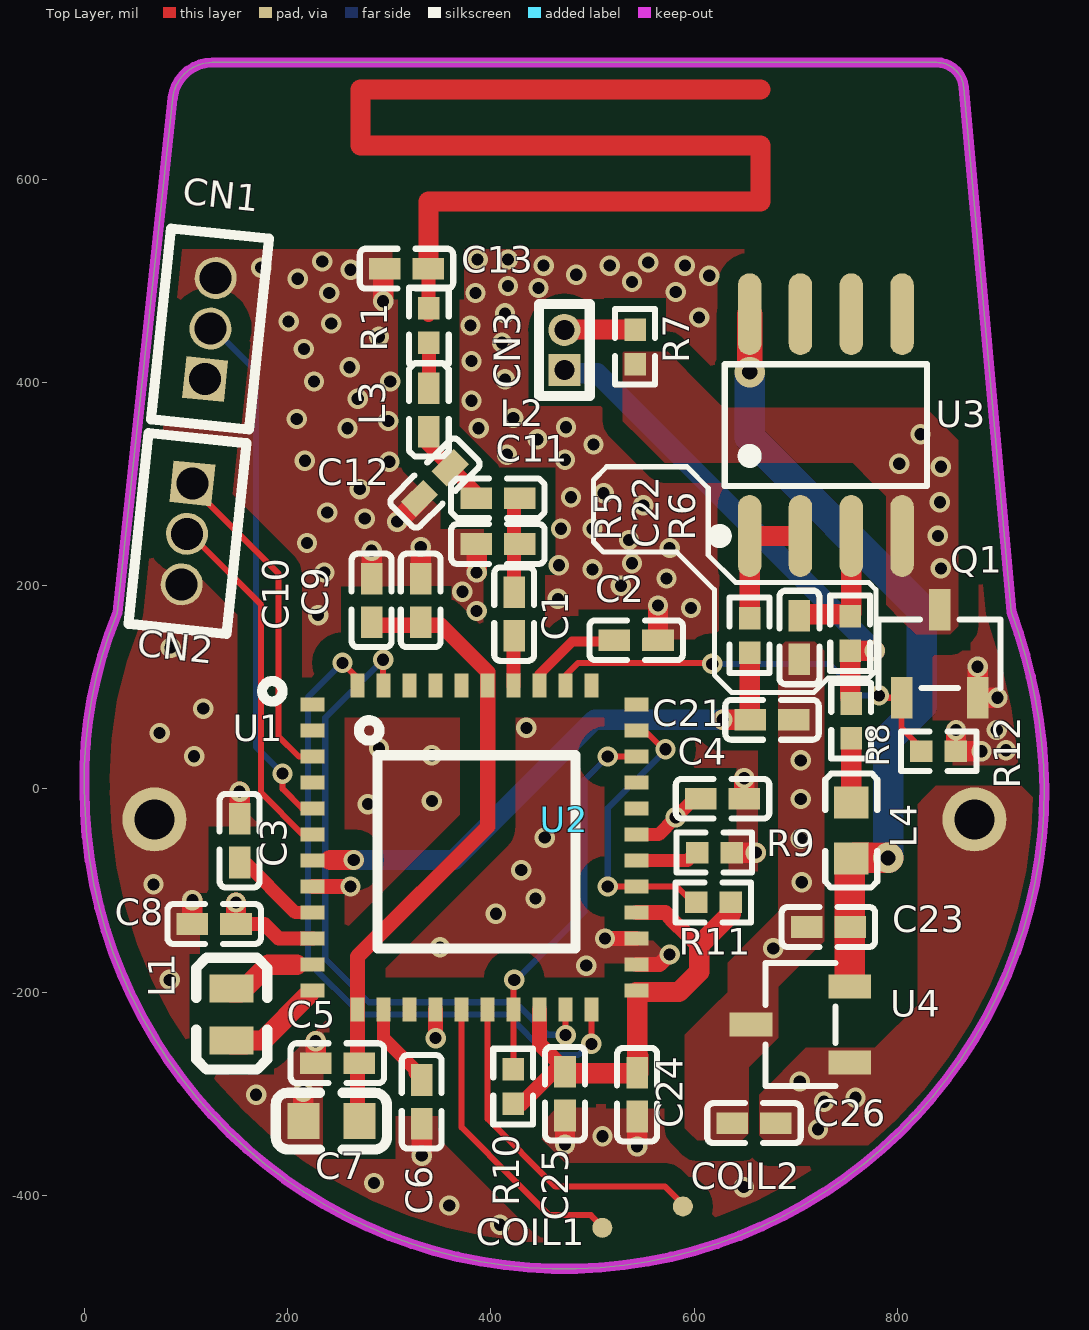
[diagram p0: Top Layer view]
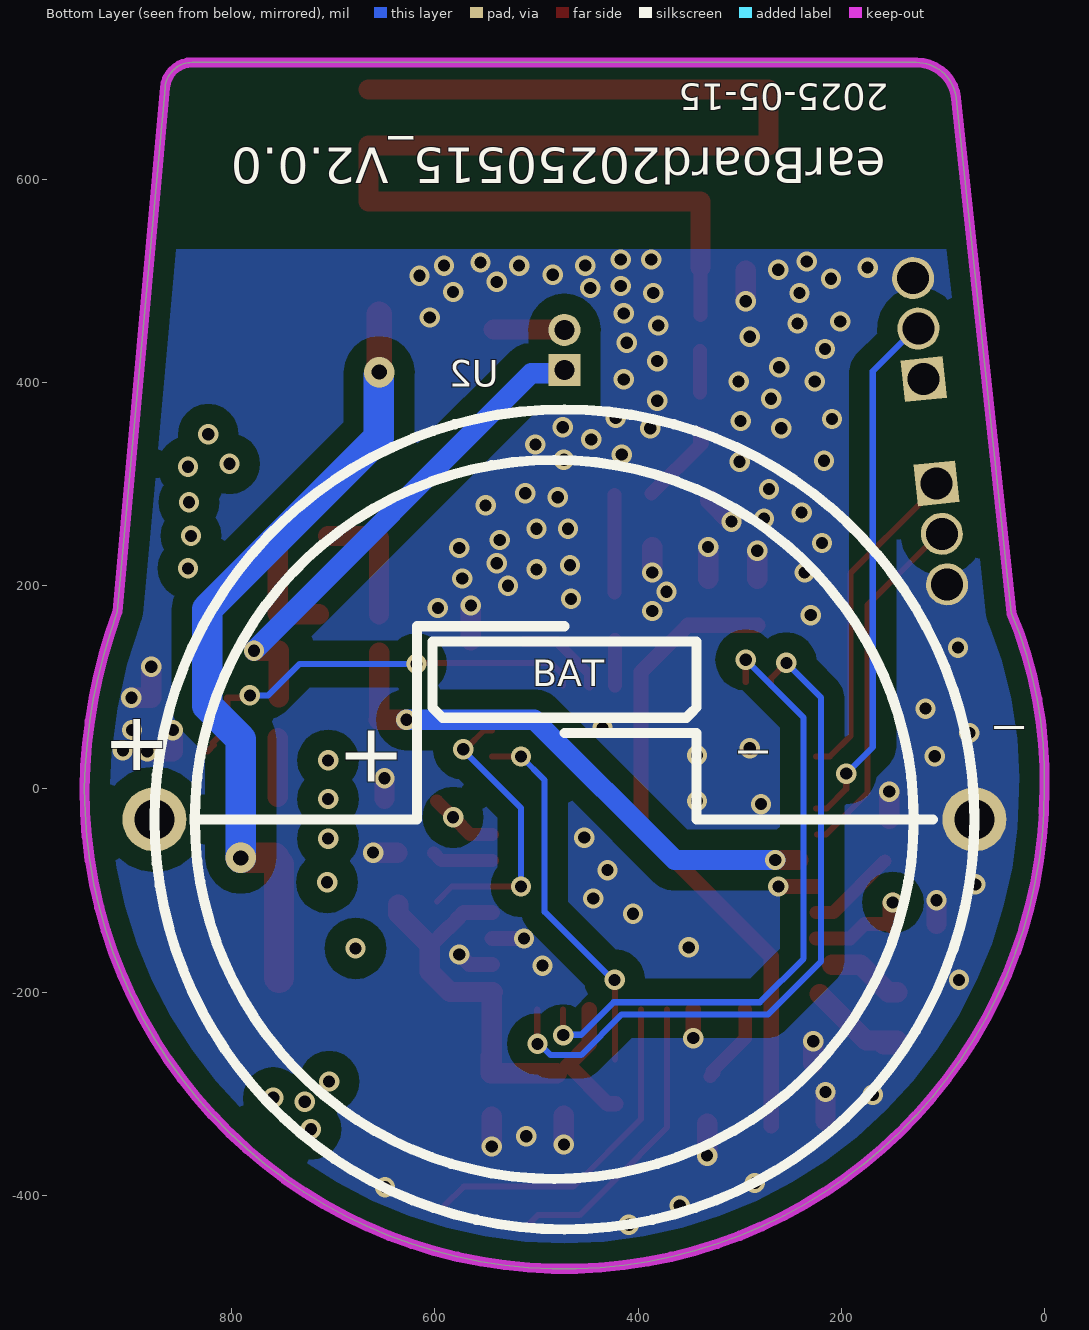
[diagram p1: Bottom Layer view, seen from below]
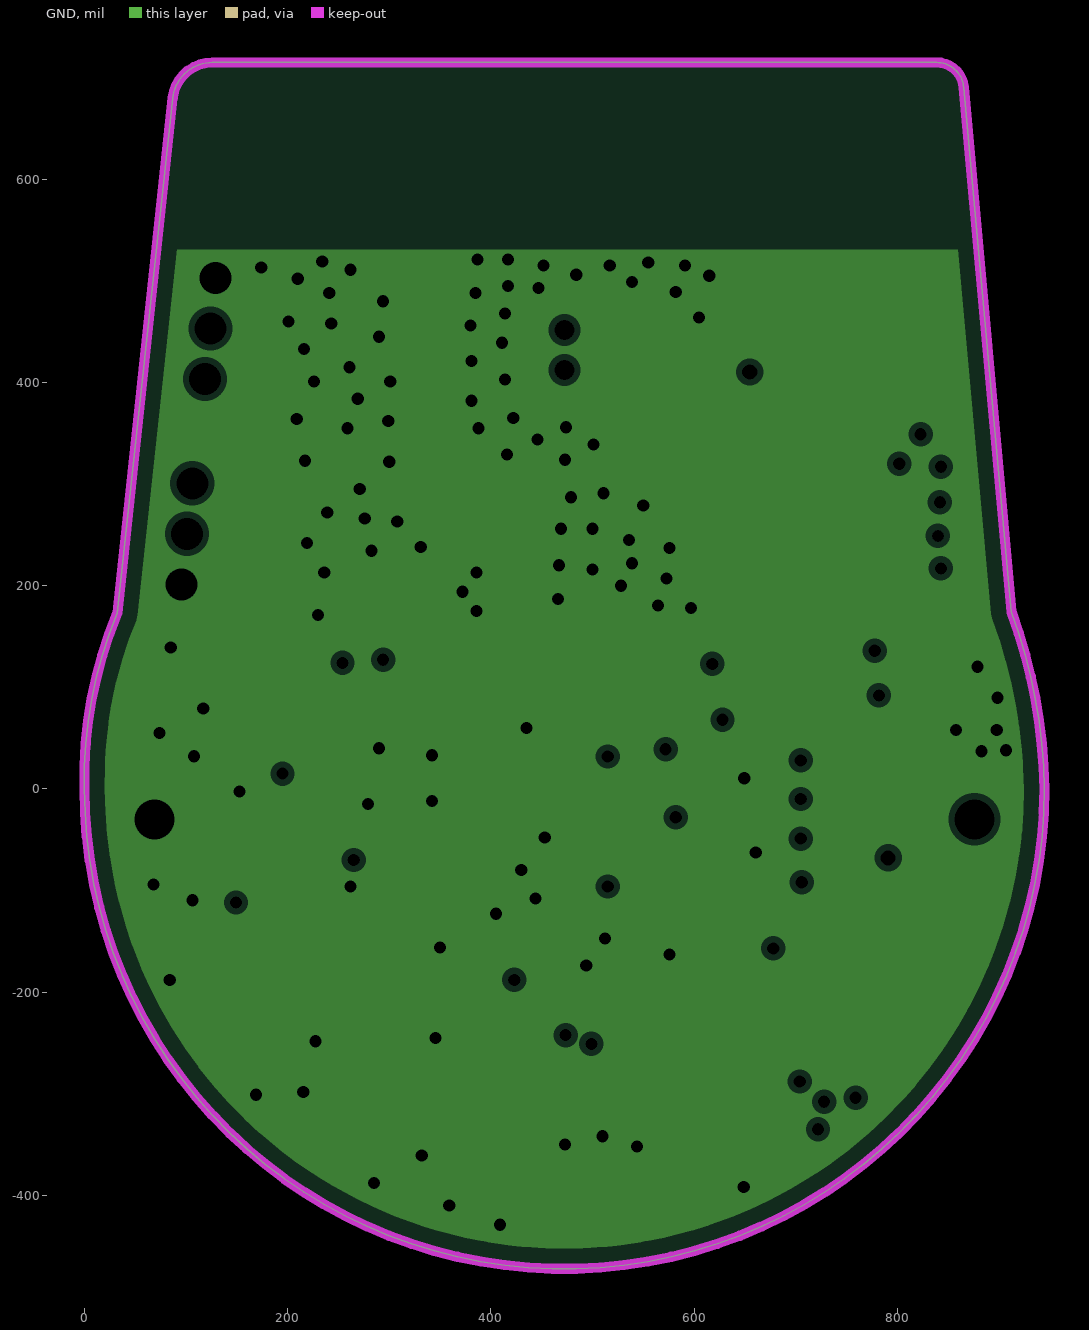
[diagram p2: GND, clearances drawn from the general rule]
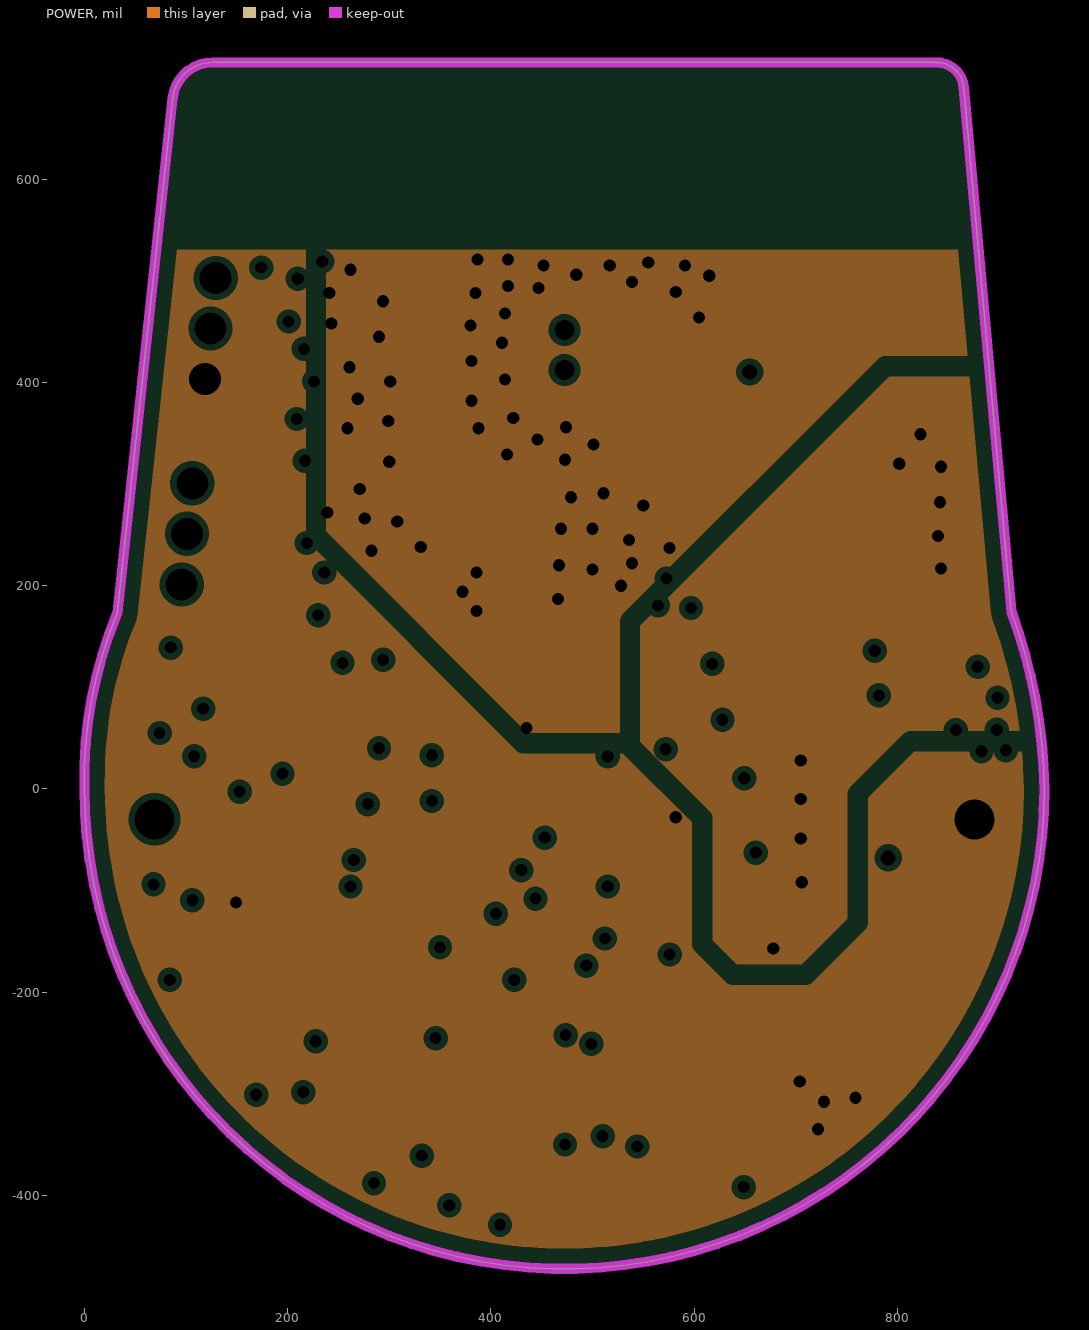
[diagram p3: POWER, clearances drawn from the general rule]
# Altium PCB MISC82703.PcbDoc
Units mil, origin at the board's own origin, x right, y up, seen from the top; angles counter-clockwise.
Board outline 944.88 x 1187.29 mil, 4 copper layers (Top Layer, GND, POWER, Bottom Layer); 42 components, 33 nets, 134 pads, 148 vias.

## Layer stack, top to bottom (the 12.6 mil dielectric is the usual default, probably not edited)
Top Layer: signal copper 1.4
Dielectric: core 12.6, FR-4, Dk 4.8
GND: plane copper 1.4, net GND
Dielectric: prepreg 12.6, FR-4, Dk 4.8
POWER: plane copper 1.4, net TL_VDD3
Dielectric: core 12.6, FR-4, Dk 4.8
Bottom Layer: signal copper 1.4

## Board outline
0,0 cw(c423.07,10.33) 32.44,173.13 86.87,679.84 cw(c126.01,675.63) 126.01,715 838.85,715 cw(c838.85,688.3) 865.48,690.34 912.44,174.28 912.44,174.29 cw(c411.43,-9.13) 944.88,0 cw(c472.44,0)

## Design rules (kind name [scope] priority, off if disabled: settings)
Clearance Clearance_1 [inpolygon] p1: gap=6
Clearance [All] p2: gap=6
DiffPairsRouting [All] p1: maxlimit=6 minlimit=6 mostfreqgap=6 maxuncoupledlength=500
HoleSize [All] p1: absolutevalues=TRUE maxlimit=500 minlimit=1 maxpercent=80.000 minpercent=20.000
HoleToHoleClearance [All] p1: gap=0 allowstackedmicrovias=TRUE
MinimumSolderMaskSliver [All] p1: minsoldermaskwidth=0
PlaneClearance [All] p1: clearance=6
PlaneConnect [All] p1: planeconnectstyle=Direct reliefexpansion=20 reliefentries=4 reliefconductorwidth=10 reliefairgap=10
PolygonConnect [All] p1: connectstyle=Direct reliefconductorwidth=10 reliefentries=4 polygonreliefangle="90 Angle"
RoutingVias [All] p1: holewidth=12 width=20 viastyle="Through Hole" minholewidth=12 minwidth=20 maxholewidth=12 maxwidth=20
SilkToSilkClearance [All] p1: silktosilkclearance=0
SilkscreenOverComponentPads [All] p1: minsilkscreentomaskgap=0
SolderMaskExpansion [All] p1: expansion=4
Width [All] p1: maxlimit=40 minlimit=6 preferedwidth=10
20 further rules are at their usual default settings.

## Classes and differential pairs
component class 1_Power电源管理+天线+加速度: C1 C2 C3 C4 C5 C6 C7 C8 C9 C10 C11 C12 C13 C24 C25 CN1 CN2 COIL1 COIL2 L1 L2 L3 R1 R9 R10 R11 U1 U2
component class 2_温度采集: C21 C22 C23 C26 CN3 L4 Q1 R5 R6 R7 R8 R12 U3 U4

## Components (designator, comment, footprint, x,y, rotation, side; value= is the part's Value field where it differs from the comment)
C1 "220pF" C0402 423,172 r90 top
C2 "1uF" C0402 543.07,146.26 r180 top
C3 "1uF" C0402 152.74,-50.99 r270 top
C4 "1uF" C0402 628.07,-9.74 r180 top
C5 "1uF" C0402 249,-270 r0 top
C6 "1uF" C0402 332,-308 r90 top
C7 "0.1uF" C0603 243,-327 r0 top
C8 "1uF" C0402 127.74,-132.99 r180 top
C9 "2.2uF" C0402 331,185.46 r270 top
C10 "0.1uF" C0402 282.7,185.45 r270 top
C11 "2pF" C0402 407,241 r0 top
C12 "2pF" C0402 345,301 r45 top
C13 "2pF" C0402 317,512 r0 top
C21 "10pF" C0402 676.74,68.01 r180 top
C22 "100nF" C0402 703.74,149.01 r90 top
C23 "100nF" C0402 732.25,-135.92 r180 top
C24 "0.1uF-c0402" C0402 544,-301 r270 top
C25 "0.1uF-c0402" C0402 473,-300 r270 top
C26 "470nF" C0402 659,-329 r0 top
CN1 "" HDR-TH_3P-P1.27-V-M-A 124,453 r84 top
CN2 "" HDR-TH_3P-P1.27-V-M-A 101,251 r264 top
CN3 "HX PZ1.0-1x2P ZZ" HDR-TH_2P-P1.00-V-M 472.44,432.01 r90 top
COIL1 "" Test-Point-0.5mm 509.74,-431.99 r0 top
COIL2 "" Test-Point-0.5mm 589,-411 r0 top
L1 "4.7uH" IND-SMD_L1.8-W1.2 145,-222 r90 top
L2 "2.4nH" L0402 407,286 r180 top
L3 "2.4nH" L0402 339,373 r90 top
L4 "MPZ1608S101ATAH0" L0603 754.74,-40.99 r270 top
Q1 "BSS138" SOT-23-3_L3.0-W1.7-P0.95-LS2.9-BR 841.74,133.01 r270 bottom
R1 "" R0402 339,456 r90 top
R5 "" R0402 654.74,151.01 r90 top
R6 "" R0402 753.74,153.01 r90 top
R7 "" R0402 542,435 r90 top
R8 "" R0402 754.74,67.01 r270 top
R9 "" R0402 620.07,-62.74 r180 top
R10 "" R0402 422,-293 r270 top
R11 "" R0402 619.07,-111.74 r0 top
R12 "" R0402 840.74,37.01 r180 top
U1 "" KTYATR0101 384.07,-57.74 r0 top
U2 "Q&J CR2032 20-6*9" BAT-TH_CR2032 472.44,-30 r180 top locked
U3 "MCP6022-I/SN" SOIC-8_L4.9-W3.9-P1.27-LS6.0-BL 729.74,358.01 r0 top
U4 "REF3025AIDBZR" SOT-23-3_L2.9-W1.6-P1.90-LS2.8-BR 704.74,-231.99 r0 bottom

## Footprints (in the part's own frame and the unit in brackets; to place one, negate y for a bottom-side part, rotate by r counter-clockwise, add the part's x,y. Pads: shape width x height; smd on the part's side, far side on the other; paste and mask are expansions set on the pad)
BAT-TH_CR2032 [mm]
  round 1.6 hole 1: 1(-10.25,0) 2(10.25,0)
C0402 [mm]
  rect 0.79x0.54 smd paste-100 mask+0.051: 1(-0.545,0) 2(0.545,0)
  silkscreen extent -1.17,-0.5 1.17,0.5
C0603 [mm]
  rect 0.8x0.9 smd: 1(-0.7,0) 2(0.7,0)
  silkscreen extent -1.39,-0.71 1.39,0.71
HDR-TH_2P-P1.00-V-M [mm]
  rect 0.8x0.8 hole 0.5 paste+0 mask+0.05: 1(-0.5,0)
  round 0.8 hole 0.5 paste+0 mask+0.05: 2(0.5,0)
  silkscreen extent -1.15,-0.64 1.15,0.64
HDR-TH_3P-P1.27-V-M-A [mm]
  rect 1.05x1.05 hole 0.8: 1(-1.27,0)
  round 1.05 hole 0.8: 2(0,0) 3(1.27,0)
  silkscreen extent -2.41,-1.22 2.39,1.24
IND-SMD_L1.8-W1.2 [mm]
  rect 0.7x1.1 smd: 1(-0.653,0) 2(0.653,0)
  silkscreen extent -1.38,-0.89 1.41,0.89
KTYATR0101 [mm]
  rect 0.6x0.35 smd: 1(-4.05,3.575) 2(-4.05,2.925) 3(-4.05,2.275) 4(-4.05,1.625) 5(-4.05,0.975) 6(-4.05,0.325) 7(-4.05,-0.325) 8(-4.05,-0.975) 9(-4.05,-1.625) 10(-4.05,-2.275) 11(-4.05,-2.925) 12(-4.05,-3.575) 23(4.05,-3.575) 24(4.05,-2.925) 25(4.05,-2.275) 26(4.05,-1.625) 27(4.05,-0.975) 28(4.05,-0.325) 29(4.05,0.325) 30(4.05,0.975) 31(4.05,1.625) 32(4.05,2.275) 33(4.05,2.925) 34(4.05,3.575)
  rect 0.35x0.6 smd: 13(-2.925,-4.05) 14(-2.275,-4.05) 15(-1.625,-4.05) 16(-0.975,-4.05) 17(-0.325,-4.05) 18(0.325,-4.05) 19(0.975,-4.05) 20(1.625,-4.05) 21(2.275,-4.05) 22(2.925,-4.05) 35(2.925,4.05) 36(2.275,4.05) 37(1.625,4.05) 38(0.975,4.05) 39(0.325,4.05) 40(-0.325,4.05) 41(-0.975,4.05) 42(-1.625,4.05) 43(-2.275,4.05) 44(-2.925,4.05)
  silkscreen extent -5.31,-2.52 2.53,4.16
L0402 [mm]
  rect 0.79x0.54 smd paste-100 mask+0.051: 1(-0.545,0) 2(0.545,0)
  silkscreen extent -1.17,-0.5 1.17,0.5
L0603 [mm]
  rect 0.8x0.864 smd paste-100 mask+0.051: 1(-0.7,0) 2(0.7,0)
  silkscreen extent -1.42,-0.65 1.42,0.65
R0402 [mm]
  rect 0.566x0.54 smd paste-100 mask+0.051: 1(-0.433,0) 2(0.433,0)
  silkscreen extent -0.94,-0.5 0.94,0.5
SOIC-8_L4.9-W3.9-P1.27-LS6.0-BL [mm]
  oval 0.588x2.045 smd: 1(-1.905,-2.772) 2(-0.635,-2.772) 3(0.635,-2.772) 4(1.905,-2.772) 5(1.905,2.772) 6(0.635,2.772) 7(-0.635,2.772) 8(-1.905,2.772)
  silkscreen extent -2.8,-2.92 2.53,1.52
SOT-23-3_L2.9-W1.6-P1.90-LS2.8-BR [mm]
  rect 1.07x0.6 smd far side: 1(1.235,0.95) 2(1.235,-0.95) 3(-1.235,0)
SOT-23-3_L3.0-W1.7-P0.95-LS2.9-BR [mil]
  rect 40.85x20.95 smd far side: 1(43.36,37.4) 2(43.36,-37.4) 3(-43.36,0)
Test-Point-0.5mm [mm]
  round 0.5 smd: 1(0,0)

## Part data
C1: library part CC0402KRX7R9BB221
C2 C3 C4 C5 C6 C8 C9 C10: library part CL05A105KA5NQNC
C7: library part CAP_0603
C11 C12 C13: library part CC0402CRNPO9BN2R0
C21: library part CC0402JRNPO9BN100
C22 C23: library part GRM155R71H104KE14D
C26: library part CGA0402X7R474K100GT
CN1 CN2: library part 3Pin_1.27___
COIL1 COIL2: library part Test-Point
L1: library part SLC1608F4R7KTT
L2 L3: library part LQG15HH2N4S02D
R1: library part SCR0402J0R
R5: library part RC0402FR-0733RL
R6 R7: library part RT0402BRD0710KL
R8: library part RT0402BRD07100KL
R9 R10 R11: library part 0402WGF4701TCE
R12: library part 0402WGF1002TCE
U1: library part KTYATR0101

## Via types
v1: diameter 20, hole 12, Top Layer to Bottom Layer, tented bottom, 105 vias
v2: diameter 20, hole 12, Top Layer to Bottom Layer, 41 vias
v3: diameter 30, hole 15, Top Layer to Bottom Layer, tented bottom, 2 vias

## Nets (pads, with @x,y where several pads share a name; then routed paths per layer and width w, separated by ;. In a path a pad name is that pad's centre, name@x,y a point inside that pad or via, vN(x,y) a via of type N, cw(c..) or ccw(c..) an arc to the next point about the centre after c; other vN are vias at no path point)
ANT: C1.1 U1.38 | length 44.8
  Top Layer w13.75: U1.38 C1.1@422.45,146.55
ANTENNA: C13.2 R1.2 | length 1334.8
  Top Layer w13.75: R1.2@338.46,466.54 C13.2
  Top Layer w19.68: C13.2@338.51,513.26 338.51,578.22 665.29,578.22 665.29,633.34 271.59,633.34 271.59,688.46 665.29,688.46
GND: C2.1 C3.1 C4.1 C5.1 C6.1 C7.1 C8.2 C9.1 C10.1 C11.1 C12.1 C13.1 C24.2 C25.2 CN1.3 CN2.3 Q1.2 R9.1 R12.1 U1.8 U1.16 U1.24 U1.25 U2.2 | length 640.2
  Top Layer w15: U1.8 v1(261.88,-96.12) ; v1(345.68,-245.32) U1.16 ; v1(512.3,-147.3) U1.25 ; U1.24 566.1,-172.9 v1(576,-163)
  Top Layer w20: C8.2 v1(106.28,-109.72) ; C3.1 v1(152.74,-2.74) ; C7.1 v1(215.44,-298.44) ; C5.1 v1(227.54,-248.46) ; C10.1 v1(282.7,234.3) ; v1(294,480) C13.1@294,510 ; v1(308,263) C12.1@329,284 ; C9.1 v1(331,238) ; v1(332,-361) C6.1 ; v1(386,213) C11.1@386,238 ; v1(473,-350) C25.2 ; v1(544,-352) C24.2 ; C2.1 v1(564.53,180.47) ; R9.1 v1(660.74,-62.74) ; C4.1 v1(649.53,10.53) ; v1(857.78,57.78) R12.1 v1(882.99,37.01) ; v1(879.14,120.14) Q1.2 v1(898.65,89.65)
  other v1: 409,-429 359,-410 649,-392 285,-388 510,-342 169,-301 84,-188 494,-174 350,-156 405,-123 444,-108 68,-94 430,-80 453,-48 279,-15 342,-12 108,32 342,33 907,38 290,40 74,55 898,58 435,60 117,79 85,139 230,171 386,175 597,178 466,187 372,194 528,200 236,213 576,237 536,245 469,256 239,272 550,279 511,291 300,322 217,323 259,355 299,362 226,401 301,401 243,458 201,460 605,464 210,502 452,515 517,515 591,515
  other v2: 573,207 500,216 467,220 539,222 219,242 500,256 276,266 479,287 271,295 473,324 416,329 501,339 446,344 388,355 474,356 209,364 422,365 381,382 269,384 414,403 261,415 381,421 216,433 411,439 290,445 380,456 414,468 241,488 385,488 582,489 447,493 417,495 539,499 615,505 484,506 262,511 174,513 555,518 234,519 387,521 417,521
NetC1_2: C1.2 C11.2 L2.1 | length 95.5
  Top Layer w13.75: C1.2 L2.1@423,289
NetC3_2: C3.2 U1.9 | length 88.6
  Top Layer w13: C3.2@157,-71 207.71,-121.71 U1.9
NetC12_2: C12.2 L2.2 L3.1 | length 76.5
  Top Layer w13.75: L3.1@337,340 L2.2@386.5,290.5 ; L3.1@339,343 L3.1@339,349.54
NetC21_1: C21.1 C22.1 C23.2 C26.1 Q1.3 R7.1 U3.4 U4.3
  other v1: 678,-157 706,-92 705,-49 705,-10 705,28 843,217 840,249 842,282 843,317 802,320 823,349
NetC22_2: C22.2 R6.2 U3.3 | length 117.2
  Top Layer w20: C22.2@714,172 754,172 754.74,172.74 U3.3
NetC23_1: C23.1 L4.2 U3.8 U4.2 | length 766.2
  Top Layer w20: L4.2@753.37,-74.63 L4.2@753.37,-71.63
  Top Layer w25: v3(654.74,410.26) U3.8
  Top Layer w30: U4.2@753.37,-186 L4.2@753.37,-74.63 ; L4.2@758,-68 v3(791,-68)
  Bottom Layer w20: v3@654.74,407 v3(654.74,410.26)
  Bottom Layer w30: v3@655,407 655,346 824,177 824,82 791,49 v3(791,-68)
NetCN3_1: CN3.1 R6.1 R8.1 | length 482
  Top Layer w20: R8.1@753.74,90.26 R6.1 v1(777.97,135.97)
  Bottom Layer w20: CN3.1@479,409 504.94,409 v1(777.97,135.97)
NetCN3_2: CN3.2 R7.2 | length 68
  Top Layer w20: CN3.2@474.04,452.04 R7.2
NetCOIL1_1: COIL1.1 U1.17 | length 296.7
  Top Layer w6: U1.17 371.27,-333.27 425,-387 457.5,-419.5 498.5,-419.5 COIL1.1@511,-432
NetCOIL2_1: COIL2.1 U1.18 | length 336.1
  Top Layer w6: U1.18 396.86,-324.86 463.5,-391.5 571.5,-391.5 COIL2.1@590,-410
NetL1_1: L1.1 U1.12 | length 108.2
  Top Layer w20: L1.1@145,-251.69 L1.1@158.31,-251.69 ; L1.1 175.31,-247.69 U1.12@221,-202
NetL1_2: L1.2 U1.11 | length 75.3
  Top Layer w20: L1.2@145,-200.31 153.69,-200.31 181,-173 209,-173
NetL3_2: L3.2 R1.1 | length 41
  Top Layer w13.75: L3.2@339,390 R1.1@339,430.96
NetL4_1: L4.1 R8.2 | length 57.7
  Top Layer w20: L4.1@754.74,-7.74 R8.2
NetR5_2: R5.2 U3.1 U3.2 | length 125.3
  Top Layer w20: R5.2@655,172 655,246.72 657.14,248.86 U3.2
NetR9_2: R9.2 U1.28 | length 60.6
  Top Layer w13: U1.28 593.47,-70.53 R9.2@601,-63
PD3: U1.21 U1.43 | length 632.6
  Top Layer w6: U1.43@294,105 v1(294,127) ; v1(473.64,-242.36) U1.21
  Bottom Layer w6: v1(294,127) 237,70 237,-167 280,-210 424,-210 456,-242 v1@473,-242 ; v1@473.14,-241.86 v1(473.64,-242.36)
PD4: U1.22 U1.44 | length 688.6
  Top Layer w6: v1(254,124) 268.91,109.09 U1.44 ; v1@499.21,-251 U1.22
  Bottom Layer w6: v1(254,124) 220,90 220,-170 272,-222 416,-222 456,-262 486,-262 v1@496,-252
  other v1: 499,-251
PGS: Q1.1 R12.2 U1.36 | length 420.6
  Top Layer w6: U1.36 473.64,111.64 486,124 v1@617,124 ; v1@780.35,89.65 Q1.1 804.34,59.66 R12.2@819,45 ; v1@780.35,92 v1(782,92) ; R12.2@817.36,43.36 R12.2
  Bottom Layer w6: v1(618,123) 733,123 764,92 v1(782,92)
RX: CN2.2 U1.6 | length 338.2
  Top Layer w6: CN2.2@113,242 174,181 174,-4 215,-45 U1.6@224,-45
SCL_ACC: R11.1 U1.27 U1.33 | length 285
  Top Layer w6: v1(515.12,-96.12) U1.27 583.12,-96.12 R11.1@598,-111 ; U1.33 551.58,57.42 568,41 v1@574,41
  Bottom Layer w6: v1(515.12,-96.12) 515.12,-18.88 572,38 v1(572,39)
SDA_ACC: R10.1 U1.19 U1.32 | length 359.9
  Top Layer w6: R10.1@422.45,-266.45 U1.19 v1@422.45,-193.55 ; v1(515.17,31.83) U1.32
  Bottom Layer w6: v1(423,-188) v1@426,-185 ; v1@427,-186 492,-121 492,8.66 v1(515.17,31.83)
TEMPA: C21.2 R5.1 U1.7 | length 530.7
  Top Layer w20: 242,-70 v1(265,-70) ; v1(628.01,68.01) C21.2 ; C21.2@654.74,73.74 R5.1
  Bottom Layer w20: v1(265,-70) 364,-70 502.01,68.01 v1(628.01,68.01)
TL_1V4: C5.2 C7.2 C9.2 C10.2 U1.13 U1.39 | length 634
  Top Layer w15: C7.2@268.91,-331.91 U1.13 268.91,-165.09 397,-37 397,115 351,161 C10.2@282,161
TL_RST: C2.2 U1.37 | length 88.5
  Top Layer w10: U1.37 448.05,113.05 480,145 C2.2@512,145
TL_SWS_A7: CN1.2 U1.5 | length 612.1
  Top Layer w6: v1(195,15) 195,0 214.35,-19.35 U1.5
  Bottom Layer w6: CN1.2@136,444 169,411 169,95 ; 169,201 169,95 ; v1(195,15) 169,41 169,95
TL_VDD3: C4.2 C8.1 C26.2 CN1.1 U1.10 U1.29 U2.1 U4.1 | length 166.3
  Top Layer w13: U1.29 565.06,-44.94 v1@581,-29 ; v1(582,-28) v1@581,-29 ; C4.2@598,-12 v1@581,-29
  Top Layer w14: C8.1@155,-133 177,-133 191.3,-147.3 U1.10
  Top Layer w20: C8.1 v1(149.2,-111.8)
  other v1: 722,-335 728,-308 759,-304 704,-288
TX: CN2.1 U1.3 | length 303.8
  Top Layer w6: CN2.1@119,284 191,212 191,52 211.17,31.83 U1.3
VDD_1V8: C6.2 U1.14 | length 79.4
  Top Layer w13: U1.14 294.5,-245.5 C6.2@327,-278 ; U1.14@295,-217.19 U1.14@295,-217 ; C6.2@325.5,-279.5 C6.2@329,-283
VDD_ACC: C24.1 C25.1 R10.2 R11.2 U1.20 U1.23 U1.26 | length 509.4
  Top Layer w15: R10.2 429.96,-310.04 467,-273 470,-273 448.05,-251.05 U1.20 ; U1.26 571.71,-121.71 577.39,-127.39 577.39,-127.96 585.3,-135.87 585.87,-135.87 605,-155
  Top Layer w20: C25.1@480,-280 543,-280 544,-279 U1.23@544,-204 ; U1.23@543,-200 585,-200 605,-180 605,-155 605,-154 636,-123 R11.2@636,-114 ; C24.1@545,-280 545,-263
pads on no net: U1.1 U1.2 U1.4 U1.15 U1.30 U1.31 U1.34 U1.35 U1.40 U1.41 U1.42 U3.5 U3.6 U3.7

## Polygon pours and split planes (outlines as drawn)
NetC21_1 on Top Layer "Bottom Layer-No Net" (solid, remove dead copper, pour order 1000): 591,-276 591,-334 596,-339 603,-346 615,-346 647,-346 652,-341 654,-339 654,-332 654,-274 679,-249 683,-245 683,-225 683,-195 723,-155 728,-150 728,-133 728,136 722,142 719,145 708,145 690,145 684,139 683,138 683,77 683,-121 654,-150 633,-171 633,-190 633,-200 618,-215 591,-242 591,-276
NetC21_1 on Top Layer "Bottom Layer-No Net" (solid, remove dead copper, pour order 1001): 530,416 530,362 548,344 571,321 653,321 756,321 777,300 789,288 789,265 789,181 805,165 818,152 839,152 852,152 858,158 860,160 860,166 860,343 827,376 826,375 695,375 629,375 611,393 574,430 551,430 531,430 530,429 530,416
TL_VDD3 on Top Layer "Bottom Layer-No Net" (solid, remove dead copper, pour order 1002): 664,-302 664,-341 670,-347 674,-351 697,-351 865,-351 903,-313 952,-264 952,-221 952,-27 923,2 922,3 903,3 838,3 827,-8 820,-15 820,-32 820,-213 781,-252 778,-255 747,-255 710,-255 664,-301
GND on Top Layer "Bottom Layer-No Net" (solid, remove dead copper, pour order 1003): -122.43,396.1 -116.43,390.1 -116.43,-499.9 967.57,-499.9 1060.57,-406.9 1131.57,-335.9 1131.57,-307.9 1131.57,757.1 1054.57,834.1 984.57,904.1 744.57,904.1 46.57,904.1 -58.43,799.1 -113.43,744.1 -113.43,415.1
GND on Bottom Layer "Bottom Layer-No Net" (solid, remove dead copper, pour order 1004): -171.87,446.8 -171.87,-330.2 -100.87,-401.2 8.13,-510.2 337.13,-510.2 883.13,-510.2 970.13,-423.2 1063.13,-330.2 1063.13,-324.2 1063.13,865.8 983.13,945.8 945.13,983.8 881.13,983.8 4.13,983.8 -132.87,846.8 -161.87,817.8 -161.87,436.8
GND on GND (split plane): 892.43,172.46 892.54,171.88 892.57,171.28 892.68,170.83 892.73,170.37 893,169.49 893.17,168.59 893.39,168.04 893.54,167.46 893.82,166.86 899.83,149.55 905.68,130.26 910.77,110.75 915.09,91.05 918.64,71.2 921.4,51.22 923.38,31.16 924.56,11.03 924.79,-0.34 924.82,-0.34 924.86,-0.78 924.49,-18.69 923.33,-37.36 921.4,-55.96 918.71,-74.47 915.25,-92.84 911.03,-111.06 906.07,-129.09 900.36,-146.9 893.93,-164.46 886.77,-181.74 878.91,-198.71 870.35,-215.33 861.11,-231.59 851.21,-247.46 840.66,-262.9 829.48,-277.89 817.69,-292.41 805.31,-306.43 792.36,-319.92 778.87,-332.87 764.85,-345.25 750.33,-357.03 735.34,-368.21 719.9,-378.76 704.04,-388.67 687.78,-397.9 671.15,-406.46 654.18,-414.33 636.91,-421.48 619.35,-427.92 601.54,-433.63 583.51,-438.59 565.29,-442.81 546.91,-446.26 528.4,-448.96 509.8,-450.89 491.14,-452.05 472.44,-452.43 453.74,-452.05 435.08,-450.89 416.48,-448.96 397.97,-446.26 379.59,-442.81 361.37,-438.59 343.34,-433.63 325.53,-427.92 307.98,-421.48 290.7,-414.33 273.73,-406.46 257.1,-397.9 240.84,-388.67 224.98,-378.76 209.54,-368.21 194.55,-357.03 180.03,-345.25 166.01,-332.87 152.52,-319.92 139.57,-306.43 127.19,-292.41 115.4,-277.89 104.23,-262.9 93.68,-247.46 83.77,-231.59 74.53,-215.33 65.97,-198.71 58.11,-181.74 50.95,-164.46 44.52,-146.9 38.81,-129.09 33.85,-111.06 29.63,-92.84 26.17,-74.47 23.48,-55.96 21.55,-37.36 20.39,-18.69 20.02,-0.78 20.1,0 20.05,0.49 20.09,0.49 19.88,10.33 20.26,27.92 21.41,45.47 23.33,62.96 26,80.35 29.44,97.6 33.62,114.69 38.54,131.57 44.19,148.23 50.49,164.43 50.84,165.04 50.96,165.42 50.99,165.4 51.01,165.44 51.27,166.3 51.62,167.13 51.79,167.97 52.06,168.78 52.09,169 52.15,169.21 52.24,170.11 52.42,170.99 91.09,531 859.8,531
TL_VDD3 on POWER (split plane): 217.91,249 218.26,246.39 219.26,243.96 220.87,241.87 424.87,37.87 426.96,36.26 429.39,35.26 432,34.91 529.83,34.91 529.87,34.87 597.91,-33.18 597.91,-153 598.26,-155.61 599.26,-158.04 600.87,-160.13 630.87,-190.13 632.96,-191.74 635.39,-192.74 638,-193.09 710,-193.09 712.61,-192.74 715.04,-191.74 717.13,-190.13 768.13,-139.13 769.73,-137.04 770.74,-134.61 771.09,-132 771.09,-9.18 817.18,36.91 922.81,36.91 923.38,31.16 924.56,11.03 924.79,-0.34 924.82,-0.34 924.86,-0.78 924.49,-18.69 923.33,-37.36 921.4,-55.96 918.71,-74.47 915.25,-92.84 911.03,-111.06 906.07,-129.09 900.36,-146.9 893.93,-164.46 886.77,-181.74 878.91,-198.71 870.35,-215.33 861.11,-231.59 851.21,-247.46 840.66,-262.9 829.48,-277.89 817.69,-292.41 805.31,-306.43 792.36,-319.92 778.87,-332.87 764.85,-345.25 750.33,-357.03 735.34,-368.21 719.9,-378.76 704.04,-388.67 687.78,-397.9 671.15,-406.46 654.18,-414.33 636.91,-421.48 619.35,-427.92 601.54,-433.63 583.51,-438.59 565.29,-442.81 546.91,-446.26 528.4,-448.96 509.8,-450.89 491.14,-452.05 472.44,-452.43 453.74,-452.05 435.08,-450.89 416.48,-448.96 397.97,-446.26 379.59,-442.81 361.37,-438.59 343.34,-433.63 325.53,-427.92 307.98,-421.48 290.7,-414.33 273.73,-406.46 257.1,-397.9 240.84,-388.67 224.98,-378.76 209.54,-368.21 194.55,-357.03 180.03,-345.25 166.01,-332.87 152.52,-319.92 139.57,-306.43 127.19,-292.41 115.4,-277.89 104.23,-262.9 93.68,-247.46 83.77,-231.59 74.53,-215.33 65.97,-198.71 58.11,-181.74 50.95,-164.46 44.52,-146.9 38.81,-129.09 33.85,-111.06 29.63,-92.84 26.17,-74.47 23.48,-55.96 21.55,-37.36 20.39,-18.69 20.02,-0.78 20.1,0 20.05,0.49 20.09,0.49 19.88,10.33 20.26,27.92 21.41,45.47 23.33,62.96 26,80.35 29.44,97.6 33.62,114.69 38.54,131.57 44.19,148.23 50.49,164.43 50.84,165.04 50.96,165.42 50.99,165.4 51.01,165.44 51.27,166.3 51.62,167.13 51.79,167.97 52.06,168.78 52.09,169 52.15,169.21 52.24,170.11 52.42,170.99 91.09,531 217.91,531
GND on POWER (split plane): 869.35,426.09 788,426.09 785.39,425.74 782.96,424.74 780.87,423.13 529.87,172.13 528.26,170.04 527.26,167.61 526.91,165 526.91,148 526.91,55.09 436.18,55.09 238.09,253.18 238.09,531 859.8,531
NetC21_1 on POWER (split plane): 892.43,172.46 892.54,171.88 892.57,171.28 892.68,170.83 892.73,170.37 893,169.49 893.17,168.59 893.39,168.04 893.54,167.46 893.82,166.86 899.83,149.55 905.68,130.26 910.77,110.75 915.09,91.05 918.64,71.2 920.59,57.09 813,57.09 810.39,56.74 807.96,55.74 805.87,54.13 753.87,2.13 752.26,0.04 751.26,-2.39 750.91,-5 750.91,-127.82 705.82,-172.91 642.18,-172.91 618.09,-148.82 618.09,-29 617.74,-26.39 616.73,-23.96 615.13,-21.87 547.09,46.18 547.09,148 547.09,160.82 792.18,405.91 871.18,405.91

## Keep-outs
Keep-Out Layer:
  the board outline again, w10

## Other copper
GND (plane layer: these items are gaps in the copper):
  rectangle: 75,531 872,721
POWER (plane layer: these items are gaps in the copper):
  rectangle: 75,531 874,721
  lines w20: 228,542 228,249 432,45 531,45 ; 893,416 788,416 537,165 537,148 537,42 608,-29 608,-153 638,-183 710,-183 761,-132 761,-5 813,47 939,47
Multi-Layer:
  pour cut-out: 14,733 10,729 10,541 20,531 936,531 977,572 977,758 897,838 75,838 14,777

## Silkscreen, mask and mechanical layers (free items; w line width, h text height)
Top Overlay:
  lines w5: 501,243 501,293 501,304 514,317 593,317 614,296 614,230 641,203 772,203 779,196 779,116 772,109 732,109 718,95 637,95 620,112 620,196 583,233 511,233 501,243
Bottom Overlay:
  text "2025-05-15" at 153,703 h45 r180
  text "earBoard20250515_V2.0.0" at 156,643 h60 r180
Mechanical 6:
  lines w0.1: 1742.06,179.47 1773.56,179.47